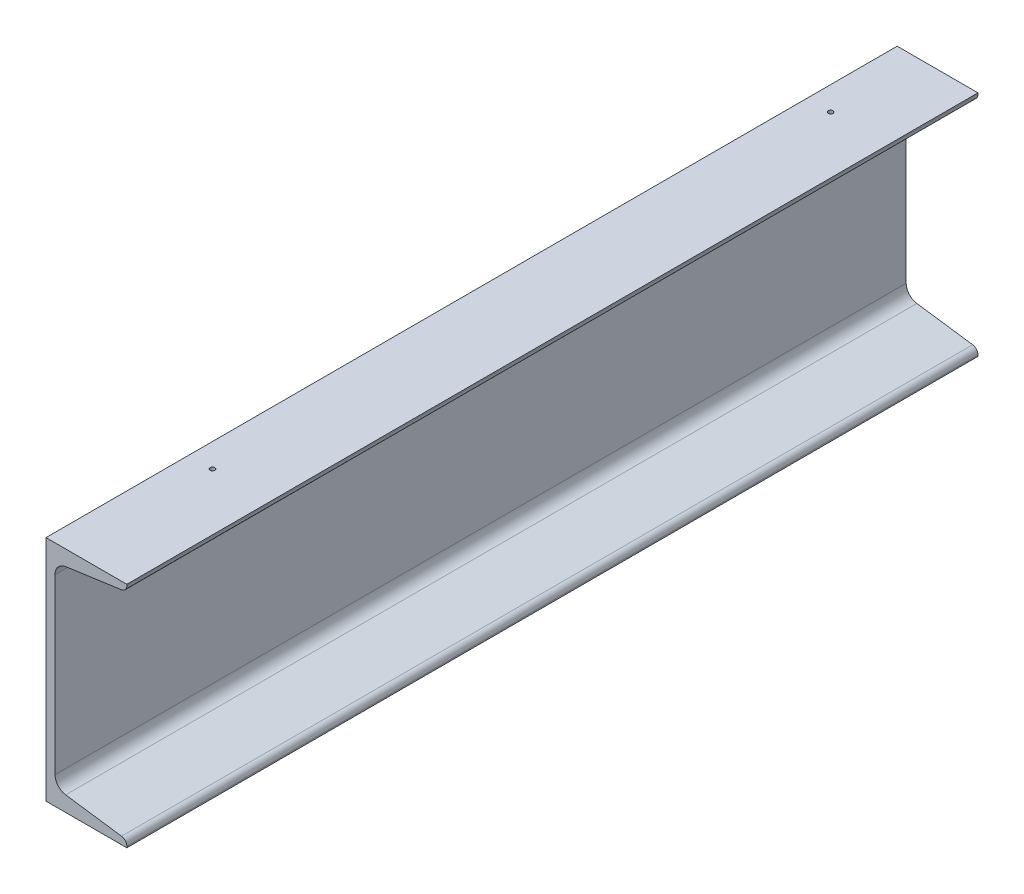
from build123d import *

# Parameters (mm, degrees)
EXTRUDE_1_DEPTH        = 895
HOLE_WIZARD_M6_1_D     = 5
HOLE_WIZARD_M6_1_DEPTH = 15
HOLE_WIZARD_M6_1_TIP   = 1.502151548


with BuildPart() as part:
    # 草图1 → 凸台-拉伸1 (new body)
    with BuildSketch(Plane.XY):
        with BuildLine():
            Line((0, 0), (-85, 0))
            Line((-85, 0), (-85, -240))
            Line((-85, -240), (0, -240))
            Line((0, -240), (0, -238.623349271))
            ThreePointArc((0, -238.623349271), (-1.594387729, -234.358965582), (-5.595374844, -232.186606824))
            Line((-5.595374844, -232.186606824), (-64.309250312, -223.934909757))
            ThreePointArc((-64.309250312, -223.934909757), (-72.311224543, -219.59019224), (-75.5, -211.061424863))
            Line((-75.5, -211.061424863), (-75.5, -28.938575137))
            ThreePointArc((-75.5, -28.938575137), (-72.311224543, -20.40980776), (-64.309250312, -16.065090243))
            Line((-64.309250312, -16.065090243), (-5.595374844, -7.813393176))
            ThreePointArc((-5.595374844, -7.813393176), (-1.594387729, -5.641034418), (0, -1.376650729))
            Line((0, -1.376650729), (0, 0))
        make_face()
    extrude(amount=EXTRUDE_1_DEPTH)

    # M6 螺纹孔1
    with Locations(Plane(origin=(0, 0, 0), x_dir=(1, 0, 0), z_dir=(0, 1, 0))):
        with Locations((-60, -745), (-60, -95)):
            Hole(HOLE_WIZARD_M6_1_D / 2, depth=HOLE_WIZARD_M6_1_DEPTH)
            with Locations((0, 0, -(HOLE_WIZARD_M6_1_DEPTH + HOLE_WIZARD_M6_1_TIP / 2))):  # 118° drill point
                Cone(0, HOLE_WIZARD_M6_1_D / 2, HOLE_WIZARD_M6_1_TIP, mode=Mode.SUBTRACT)


solid = part.part
